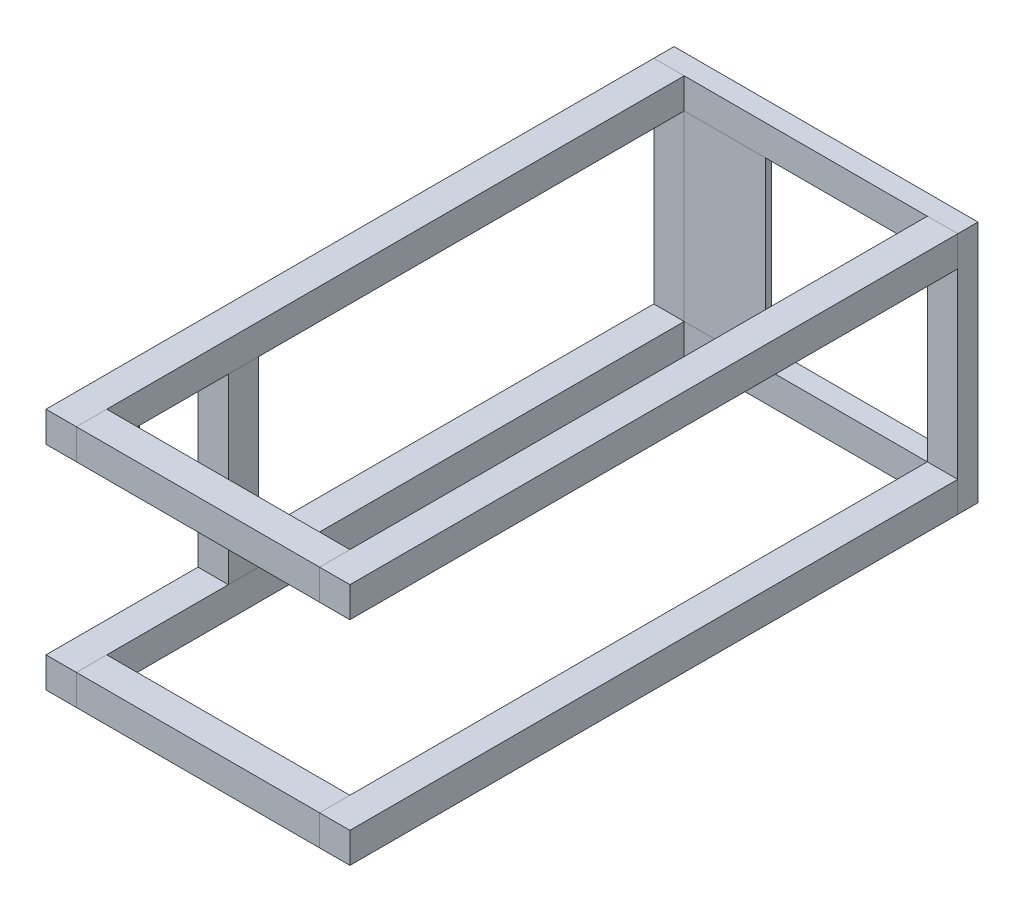
SolidWorks part; units mm, degrees
ref_plane "Front Plane" through (0, 0, 0) normal (0, 0, 1) x (1, 0, 0)
ref_plane "Top Plane" through (0, 0, 0) normal (0, 1, 0) x (1, 0, 0)
ref_plane "Right Plane" through (0, 0, 0) normal (1, 0, 0) x (0, 0, -1)
sketch "Sketch2" plane through (0, 0, 0) normal (0, 0, 1) x (1, 0, 0)
  line L1 (-75, 60) -> (75, 60)
  line L2 (-75, 60) -> (-75, -60)
  line L3 (-75, -60) -> (75, -60)
  line L4 (75, 60) -> (75, -60)
  line L5 (-75, 60) -> (75, -60) construction
  line L6 (-75, -60) -> (75, 60) construction
  point P0 (0, 0)
  dimension "D1" = 150
  dimension "D2" = 120
extrude "Boss-Extrude1" add sketch "Sketch2" along normal blind 10
sketch "Sketch6" plane through (0, 0, 10) normal (0, 0, 1) x (1, 0, 0)
  line L0 (75, -60) -> (75, 60) construction
  line L1 (-60, 45) -> (60, 45)
  line L2 (-60, 45) -> (-60, -45)
  line L3 (-60, -45) -> (60, -45)
  line L4 (60, 45) -> (60, -45)
  line L5 (-60, 45) -> (60, -45) construction
  line L6 (-60, -45) -> (60, 45) construction
  line L7 (-75, -60) -> (75, -60) construction
  point P0 (0, 0)
  dimension "D1" = 15
  dimension "D2" = 15
extrude "Cut-Extrude4" cut sketch "Sketch6" against normal through all both and the other way through all
sketch "Sketch7" plane through (0, 0, 10) normal (0, 0, 1) x (1, 0, 0)
  line L1 (-75, 60) -> (-60, 60)
  line L2 (-75, 60) -> (-75, 45)
  line L3 (-75, 45) -> (-60, 45)
  line L4 (-60, 60) -> (-60, 45)
  line L5 (-75, -60) -> (-60, -60)
  line L6 (-75, -60) -> (-75, -45)
  line L7 (-75, -45) -> (-60, -45)
  line L8 (-60, -60) -> (-60, -45)
  line L13 (75, 60) -> (60, 60)
  line L14 (75, 60) -> (75, 45)
  line L15 (75, 45) -> (60, 45)
  line L16 (60, 60) -> (60, 45)
  line L17 (75, -60) -> (60, -60)
  line L18 (75, -60) -> (75, -45)
  line L19 (75, -45) -> (60, -45)
  line L20 (60, -60) -> (60, -45)
extrude "Boss-Extrude2" add sketch "Sketch7" along normal blind 300 separate body
sketch "Sketch8" plane through (0, 0, 10) normal (0, 0, 1) x (1, 0, 0)
  line L1 (75, 60) -> (60, 60)
  line L2 (75, 60) -> (75, 45)
  line L3 (75, 45) -> (60, 45)
  line L4 (60, 60) -> (60, 45)
  line L5 (60, -45) -> (75, -45)
  line L6 (60, -45) -> (60, -60)
  line L7 (60, -60) -> (75, -60)
  line L8 (75, -45) -> (75, -60)
ref_plane "Plane1" through (0, 0, 155) normal (0, 0, 1) x (1, 0, 0)
sketch "Sketch14" plane through (-60, 0, 0) normal (1, 0, 0) x (0, 0, -1)
  line L0 (-310, 45) -> (-10, 45) construction
  line L1 (-310, 60) -> (-295, 60)
  line L2 (-310, 60) -> (-310, 45)
  line L3 (-310, 45) -> (-295, 45)
  line L4 (-295, 60) -> (-295, 45)
  line L5 (-310, -60) -> (-10, -60) construction
  line L6 (-310, -45) -> (-295, -45)
  line L7 (-310, -45) -> (-310, -60)
  line L8 (-310, -60) -> (-295, -60)
  line L9 (-295, -45) -> (-295, -60)
  dimension "D1" = 15
  dimension "D2" = 15
extrude "Boss-Extrude7" add sketch "Sketch14" along normal up to surface (120 mm away) separate body up to face at (60, -52.5, 160)
sketch "Sketch15" plane through (0, 45, 0) normal (0, -1, 0) x (1, 0, 0)
  line L0 (-75, 310) -> (-75, 10) construction
  line L1 (-75, 235) -> (-60, 235)
  line L2 (-75, 235) -> (-75, 220)
  line L3 (-75, 220) -> (-60, 220)
  line L4 (-60, 235) -> (-60, 220)
  line L5 (-60, 310) -> (-60, 10) construction
  line L6 (-75, 10) -> (-60, 10) construction
  dimension "D1" = 210
  dimension "D2" = 15
extrude "Boss-Extrude8" add sketch "Sketch15" along normal up to surface (90 mm away) separate body up to face at (-67.5, -45, 160)
sketch "Sketch16" plane through (0, 45, 0) normal (0, -1, 0) x (1, 0, 0)
  line L0 (-67.5, 310) -> (-67.5, 255.6313) construction
  line L1 (-75, 310) -> (-60, 310) construction
  circle A0 centre (-67.5, 275) radius 2.5
  dimension "D1" = 5
  dimension "D2" = 35
extrude "Boss-Extrude9" add sketch "Sketch16" along normal blind 14
sketch "Sketch17" plane through (0, 0, 10) normal (0, 0, 1) x (1, 0, 0)
  line L0 (-60, 45) -> (-60, -45) construction
  line L1 (-60, 45) -> (-20, 45)
  line L2 (-60, 45) -> (-60, -45)
  line L3 (-60, -45) -> (-20, -45)
  line L4 (-20, 45) -> (-20, -45)
  line L5 (0, 0) -> (-33.9293, 0) construction
  dimension "D1" = 40
  dimension "D2" = 90
extrude "Boss-Extrude10" add sketch "Sketch17" against normal blind 3 separate body
